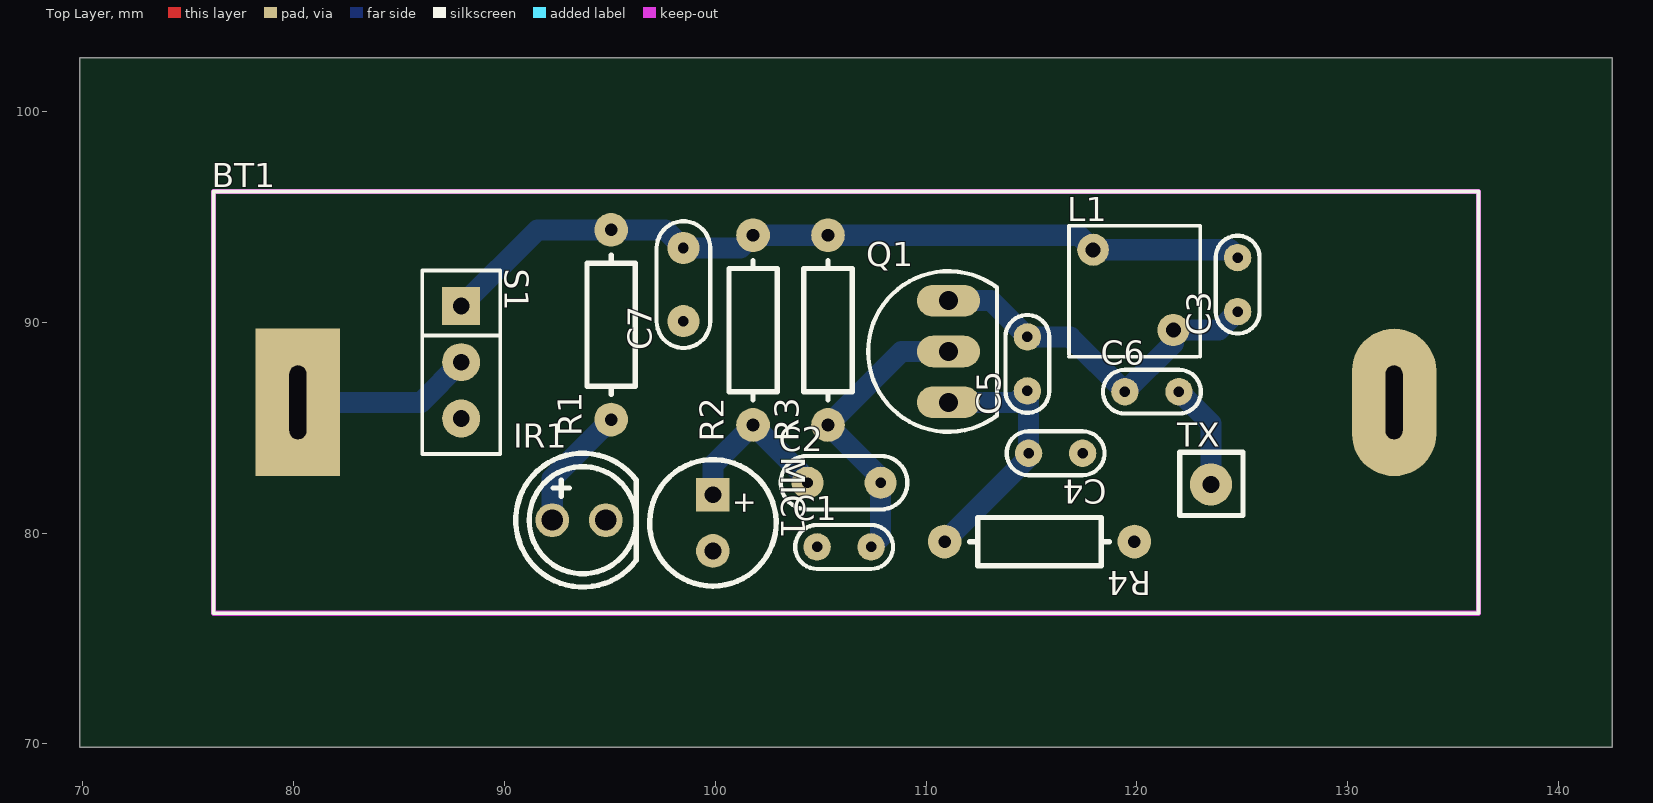
[diagram p0: Top Layer view]
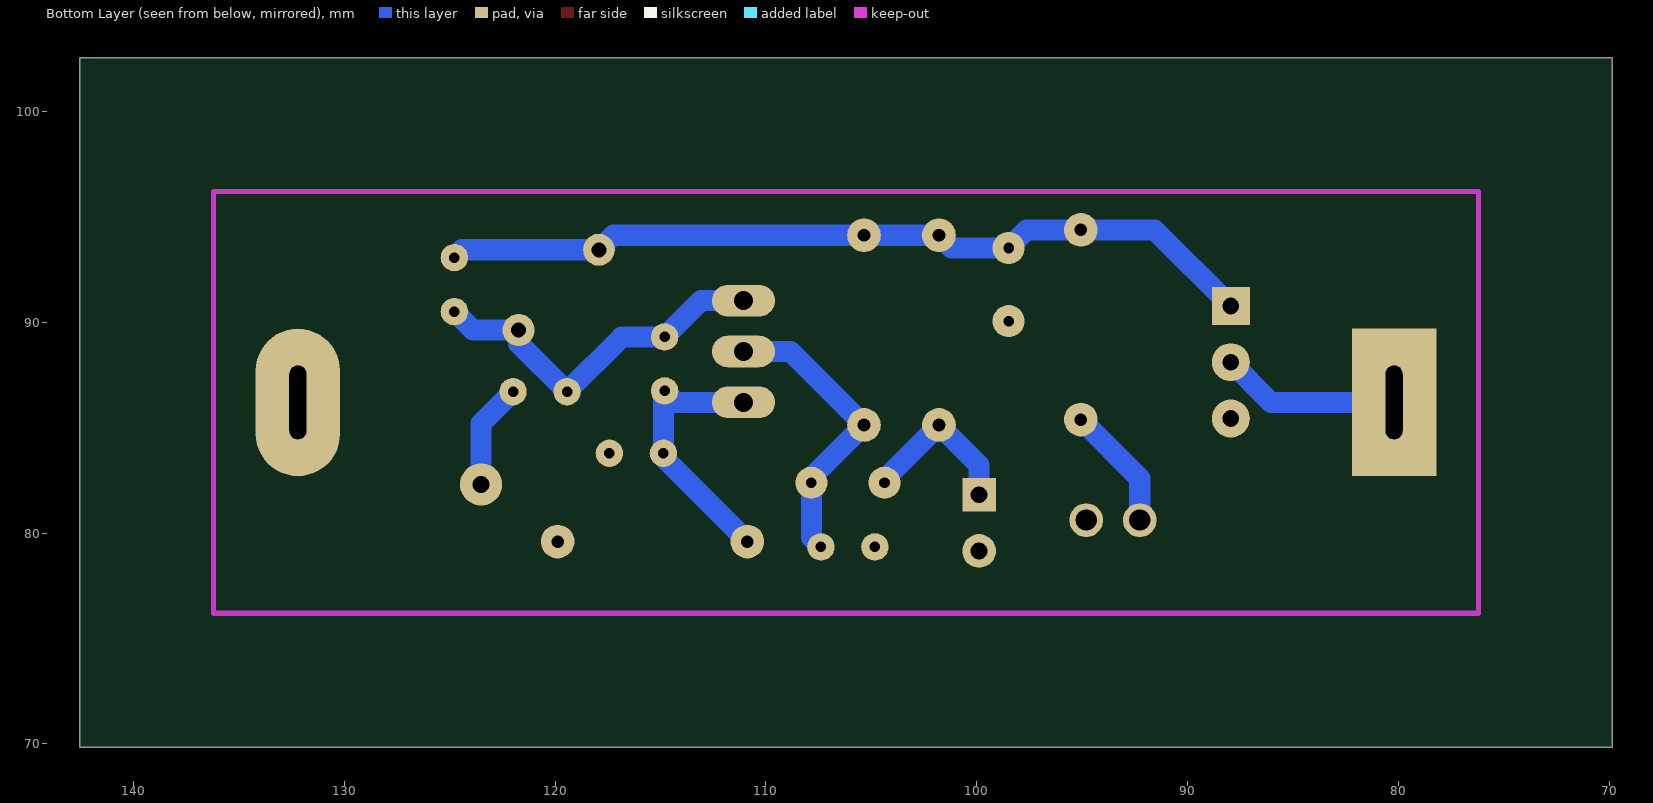
[diagram p1: Bottom Layer view, seen from below]
# Altium PCB MISC51881.pcbdoc
Units mm, origin at the board's own origin, x right, y up, seen from the top; angles counter-clockwise.
Board outline 72.7 x 32.7 mm, 2 copper layers (Top Layer, Bottom Layer), stack 1.58 mm thick; 18 components, 9 nets, 37 pads, 0 vias.

## Layer stack, top to bottom
Top Solder Mask Layer: solder mask 0.01, Dk 3.3
Top Layer: signal copper 0.035
Dielectric1: surface 1.51, FR4, Dk 4.5
Bottom Layer: signal copper 0.035
Bottom Solder Mask Layer: solder mask 0.01, Dk 3.3

## Board outline
142.55,69.85 69.85,69.85 69.85,102.55 142.55,102.55

## Design rules (kind name [scope] priority, off if disabled: settings)
BoardOutlineClearance copperThickness2oz_1 [All] p2 off: genericclearance=0.203 ignorepadtopadclearanceinfootprint=FALSE except(0: Arc-SplitContinuation Track-SplitContinuation SMDPad-SplitContinuation THPad-SplitContinuation Via-SplitContinuation Fill-SplitContinuation Region-SplitContinuation Poly-SplitContinuation Text-SplitContinuation Hole-SplitContinuation; 0.152: Arc-CutoutEdge SMDPad-CutoutEdge THPad-CutoutEdge Via-CutoutEdge Fill-CutoutEdge Region-CutoutEdge Text-CutoutEdge; 0.176: Hole-OutlineEdge Hole-CutoutEdge; 0.254: Poly-OutlineEdge Poly-CutoutEdge; 0.3: Arc-OutlineEdge Track-OutlineEdge SMDPad-OutlineEdge THPad-OutlineEdge Via-OutlineEdge Fill-OutlineEdge Region-OutlineEdge Text-OutlineEdge Track-CutoutEdge)
BoardOutlineClearance copperThickness1oz_1 [All] p4: genericclearance=0.102 ignorepadtopadclearanceinfootprint=FALSE except(0: Arc-SplitContinuation Track-SplitContinuation SMDPad-SplitContinuation THPad-SplitContinuation Via-SplitContinuation Fill-SplitContinuation Region-SplitContinuation Poly-SplitContinuation Text-SplitContinuation Hole-SplitContinuation; 0.152: SMDPad-CutoutEdge THPad-CutoutEdge Via-CutoutEdge Fill-CutoutEdge Region-CutoutEdge Text-CutoutEdge; 0.176: Hole-OutlineEdge Hole-CutoutEdge; 0.254: Poly-OutlineEdge Poly-CutoutEdge; 0.3: Arc-OutlineEdge Track-OutlineEdge SMDPad-OutlineEdge THPad-OutlineEdge Via-OutlineEdge Fill-OutlineEdge Region-OutlineEdge Text-OutlineEdge Arc-CutoutEdge Track-CutoutEdge)
Clearance copperThickness2oz [All] p1 off: gap=0.203 ignorepadtopadclearanceinfootprint=FALSE except(0.152: SMDPad-Track SMDPad-SMDPad THPad-Track SMDPad-THPad THPad-THPad Track-Via SMDPad-Via THPad-Via Via-Via Fill-Track Region-Track Fill-SMDPad Region-SMDPad Fill-THPad Region-THPad Fill-Via Region-Via Fill-Fill Fill-Region Region-Region Arc-Track Arc-SMDPad Arc-THPad Arc-Via Fill-Arc Region-Arc Arc-Arc Text-Track SMDPad-Text Text-THPad Text-Via Fill-Text Region-Text Arc-Text Text-Text; 0.176: Hole-Track Hole-SMDPad Hole-THPad Hole-Via Fill-Hole Region-Hole Hole-Arc Hole-Text; 0.254: Poly-Track Poly-SMDPad Poly-THPad Poly-Via Poly-Fill Poly-Region Poly-Poly Poly-Arc Poly-Text Poly-Hole)
Clearance copperThickness1oz [All] p3: gap=0.102 ignorepadtopadclearanceinfootprint=FALSE except(0.152: SMDPad-Track SMDPad-SMDPad THPad-Track SMDPad-THPad THPad-THPad Track-Via SMDPad-Via THPad-Via Via-Via Fill-Track Region-Track Fill-SMDPad Region-SMDPad Fill-THPad Region-THPad Fill-Via Region-Via Fill-Fill Fill-Region Region-Region Arc-Track Arc-SMDPad Arc-THPad Arc-Via Fill-Arc Region-Arc Arc-Arc Text-Track SMDPad-Text Text-THPad Text-Via Fill-Text Region-Text Arc-Text Text-Text; 0.176: Hole-Track Hole-SMDPad Hole-THPad Hole-Via Fill-Hole Region-Hole Hole-Arc Hole-Text; 0.254: Poly-Track Poly-SMDPad Poly-THPad Poly-Via Poly-Fill Poly-Region Poly-Poly Poly-Arc Poly-Text Poly-Hole)
DiffPairsRouting differentialPair [All] p1: maxlimit=0.152 minlimit=0.152 mostfreqgap=0.152 toplayer_minwidth=0.127 toplayer_prefwidth=0.254 toplayer_maxwidth=2.54 toplayer_mingap=0.152 toplayer_prefgap=0.152 toplayer_maxgap=0.152 bottomlayer_minwidth=0.127 bottomlayer_prefwidth=0.254 bottomlayer_maxwidth=2.54 bottomlayer_mingap=0.152 bottomlayer_prefgap=0.152 bottomlayer_maxgap=0.152 maxuncoupledlength=0.254
HoleToHoleClearance otherClearance [All] p1: gap=0.3 allowstackedmicrovias=TRUE
Length netLength [All] p1: minlimit=0 maxlimit=0
MatchedLengths netLengthTolerance [All] p1: tolerance=25.4
PasteMaskExpansion pasteMaskExpansion [All] p1: expansion=0
PlaneConnect innerPlane [All] p1: planeconnectstyle=Relief reliefexpansion=0.508 reliefentries=4 reliefconductorwidth=0.254 reliefairgap=0.254
PolygonConnect copperRegion [(InNet('GND'))] p1: connectstyle=Relief reliefconductorwidth=0.254 reliefentries=4 polygonreliefangle="90 Angle" airgapwidth=0.254 via.connectstyle=Relief via.reliefconductorwidth=0.254 via.reliefentries=4 via.polygonreliefangle="90 Angle" via.airgapwidth=0.254
RoutingVias viaSize [All] p1: holewidth=0.305 width=0.61 viastyle="Through Hole" minholewidth=0.3 minwidth=0.5 maxholewidth=6.3 maxwidth=10
SolderMaskExpansion solderMaskExpansion [IsVia] p1: expansion=-25.4 istentingtop=TRUE
SolderMaskExpansion solderMaskExpansion [All] p2: expansion=0.051 istentingtop=FALSE
Width copperThickness2oz_2 [All] p1 off: maxlimit=2.54 minlimit=0.203 preferedwidth=0.254
Width copperThickness1oz_2 [All] p2: maxlimit=0.254 minlimit=0.254 preferedwidth=0.254 toplayer_minwidth=0.127 toplayer_maxwidth=2.54 toplayer_prefwidth=0.254 bottomlayer_minwidth=1.001 bottomlayer_maxwidth=1.001 bottomlayer_prefwidth=1.001

## Components (designator, comment, footprint, x,y, rotation, side; value= is the part's Value field where it differs from the comment)
BT1 "BATTERY" Bat_Box_01 80.2,86.2 r0 top
C1 "103" "CC 1.8*3.6" 106.108,79.342 r0 top
C2 "104" "CC 2.2*5" 106.108,82.39 r0 top
C3 "30pf" "CC 1.8*3.6" 124.777,91.788 r90 top
C4 "30pf" "CC 1.8*3.6" 116.141,83.787 r180 top
C5 "10pf" "CC 1.8*3.6" 114.803,88.023 r90 top
C6 "30pf" "CC 1.8*3.6" 120.713,86.708 r0 top
C7 "104" "CC 2.2*5" 98.488,91.788 r90 top
IR1 "LED_R_L" LED-TH_BD5.0-P2.54-FD 93.535,80.612 r0 top
L1 "4T" IND_5x5 117.919,93.439 r0 top
MIC1 "MIC" MIC-TH_BD6.0-P1.90-D0.4-L-FD_GMI6050P-2CXXDB 99.885,80.485 r270 top
Q1 "9018" TANS 111.061,88.613 r0 top
R1 "Res" AXIAL0.4-1/4W 95.059,89.883 r90 top
R2 "Res" AXIAL0.4-1/4W 101.79,89.629 r90 top
R3 "Res" AXIAL0.4-1/4W 105.346,89.629 r90 top
R4 "Res" AXIAL0.4-1/4W 115.379,79.596 r180 top
S1 "MTS-10x" SW-TH_KH-SS12D01-G3-5.0 87.947,88.105 r270 top
TX "TX" TX 123.509,82.308 r0 top

## Footprints (in the part's own frame and the unit in brackets; to place one, negate y for a bottom-side part, rotate by r counter-clockwise, add the part's x,y. Pads: shape width x height; smd on the part's side, far side on the other; paste and mask are expansions set on the pad)
AXIAL0.4-1/4W [mm]
  round 1.6 hole 0.6: 1(-4.5,0) 2(4.5,0)
  silkscreen extent -3.3,-1.14 3.3,1.14
Bat_Box_01 [mm]
  rect 4x7 hole 0.8 slot 3.5 at 90 deg: 1(0,0)
  oval 4x7 hole 0.8 slot 3.5 at 90 deg: 2(52,0)
  silkscreen extent -4,-10 56,10
"CC 1.8*3.6" [mm]
  round 1.3 hole 0.5: 1(-1.281,0) 2(1.281,0)
  silkscreen extent -2.32,-1.04 2.32,1.04
"CC 2.2*5" [mm]
  round 1.524 hole 0.5: 1(-1.735,0) 2(1.735,0)
  silkscreen extent -3,-1.27 3,1.27
IND_5x5 [mil]
  oval 59.06x60 hole 28: 1(0,0)
  round 60 hole 28: 2(150,-150)
  silkscreen extent -45,-200 200,45
LED-TH_BD5.0-P2.54-FD [mm]
  round 1.6 hole 1: 1(-1.27,0) 2(1.27,0)
  silkscreen extent -2.99,-3.17 2.72,3.17
MIC-TH_BD6.0-P1.90-D0.4-L-FD_GMI6050P-2CXXDB [mm]
  rect 1.6x1.6 hole 0.8: 1(-1.331,0)
  round 1.6 hole 0.8: 2(1.331,0)
  silkscreen extent -3,-3 3,3
SW-TH_KH-SS12D01-G3-5.0 [mm]
  rect 1.8x1.8 hole 0.8 paste+0 mask+0.05: 1(-2.667,0)
  round 1.8 hole 0.8 paste+0 mask+0.05: 2(0,0) 3(2.667,0)
  silkscreen extent -4.35,-1.85 4.35,1.85
TANS [mm]
  oval 3x1.5 hole 0.9: 1(0,-2.413) 2(0,0) 3(0,2.413)
  silkscreen extent -3.81,-3.81 2.3,3.81
TX [mm]
  round 2 hole 0.8: 1(0,0)
  silkscreen extent -1.48,-1.48 1.52,1.52

## Nets (pads, with @x,y where several pads share a name; then routed paths per layer and width w, separated by ;. In a path a pad name is that pad's centre, name@x,y a point inside that pad or via, vN(x,y) a via of type N, cw(c..) or ccw(c..) an arc to the next point about the centre after c; other vN are vias at no path point)
1.5V: BT1.1 S1.2 | length 8.5
  Bottom Layer w1: BT1.1 86.042,86.2 S1.2
$1N8: IR1.1 R1.1 | length 5.9
  Bottom Layer w1: IR1.1 92.265,82.589 R1.1
$1N10: C2.1 MIC1.1 R2.1 | length 7.9
  Bottom Layer w1: MIC1.1 99.885,83.224 R2.1 104.373,82.546 C2.1
$1N12: C1.2 C2.2 Q1.2 R3.1 | length 14.2
  Bottom Layer w1: C1.2 107.843,79.796 C2.2 107.843,82.632 R3.1 108.83,88.613 Q1.2
$1N14: C3.1 C5.2 C6.1 L1.2 Q1.3 | length 17.4
  Bottom Layer w1: Q1.3 113.081,91.026 C5.2 116.836,89.304 C6.1 121.729,89.005 L1.2 123.899,89.629 C3.1
$1N15: C4.2 C5.1 Q1.1 R4.2 | length 12.8
  Bottom Layer w1: R4.2 114.86,83.577 C4.2 114.86,86.685 C5.1 114.261,86.2 Q1.1
$1N18: C6.2 TX.1 | length 5
  Bottom Layer w1: C6.2 123.509,85.193 TX.1
GND: BT1.2 C1.1 C4.1 C7.1 IR1.2 MIC1.2 R4.1
VCC: C3.2 C7.2 L1.1 R1.2 R2.2 R3.2 S1.1 | length 39.4
  Bottom Layer w1: S1.1 91.558,94.383 R1.2 97.628,94.383 C7.2 101.184,93.523 R2.2 R3.2 117.229,94.129 L1.1 124.407,93.439 C3.2
pads on no net: S1.3

## Keep-outs
Board Outline Layer:
  lines w0.254: 76.2,76.2 76.2,96.2 136.2,96.2 136.2,76.2 76.2,76.2